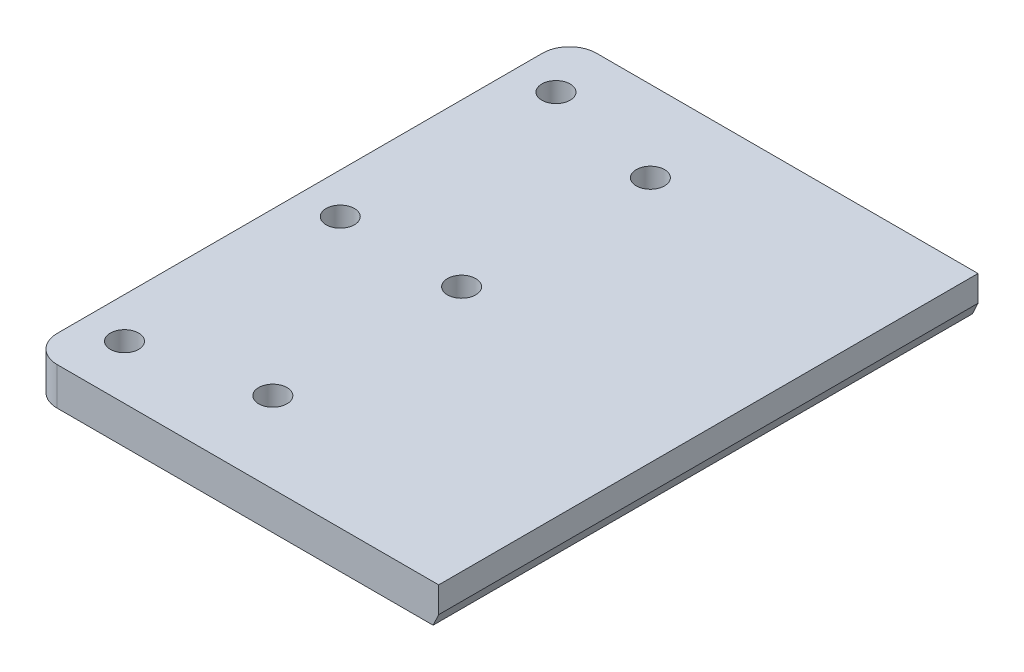
from build123d import *

# Parameters (mm, degrees)
BOSS_EXTRUDE1_DEPTH          = 14
FILLET1_R                    = 10
F_10_5_10_5_DIAMETER_HOLE1_D = 10.5
F_10_5_10_5_DIAMETER_HOLE2_D = 10.5
CUT_EXTRUDE1_DEPTH           = 257.507309837
SKETCH8_W                    = 4.462850671
SKETCH8_H                    = 15.00402921
CUT_EXTRUDE2_DEPTH           = 255.008682508


with BuildPart() as part:
    # Sketch1 → Boss-Extrude1 (new body)
    with BuildSketch(Plane(origin=(0, 0, 0), x_dir=(1, 0, 0), z_dir=(0, 1, 0))):
        Polygon((0, -100), (0, 100), (80, 100), (160, 100), (160, -100), (80, -100), align=None)
    extrude(amount=BOSS_EXTRUDE1_DEPTH)

    # Fillet1
    fillet1_edges = [part.edges().sort_by_distance(p)[0] for p in [
        (0, 7, 100),
        (0, 7, -100),
    ]]
    fillet(fillet1_edges, radius=FILLET1_R)

    # Ø10.5 (10.5) Diameter Hole1 (through all)
    with Locations(Plane(origin=(0, 14, 0), x_dir=(1, 0, 0), z_dir=(0, 1, 0))):
        with Locations((60, 70), (60, -70), (60, 0)):
            Hole(F_10_5_10_5_DIAMETER_HOLE1_D / 2)

    # Ø10.5 (10.5) Diameter Hole2 (through all)
    with Locations(Plane(origin=(0, 14, 0), x_dir=(1, 0, 0), z_dir=(0, 1, 0))):
        with Locations((15, 80), (15, -80), (15, 0)):
            Hole(F_10_5_10_5_DIAMETER_HOLE2_D / 2)

    # Sketch7 → Cut-Extrude1 (cut, through all)
    with BuildSketch(Plane.XY.offset(100)):
        Polygon((149.434543456, 0), (160, 22.657694676), (160, 0), align=None)
    extrude(amount=-CUT_EXTRUDE1_DEPTH, mode=Mode.SUBTRACT)

    # Sketch8 → Cut-Extrude2 (cut, through all)
    with BuildSketch(Plane.XY.offset(100)):
        with Locations((153.731425336, 6.497985395)):
            Rectangle(SKETCH8_W, SKETCH8_H)
    extrude(amount=-CUT_EXTRUDE2_DEPTH, mode=Mode.SUBTRACT)


solid = part.part
